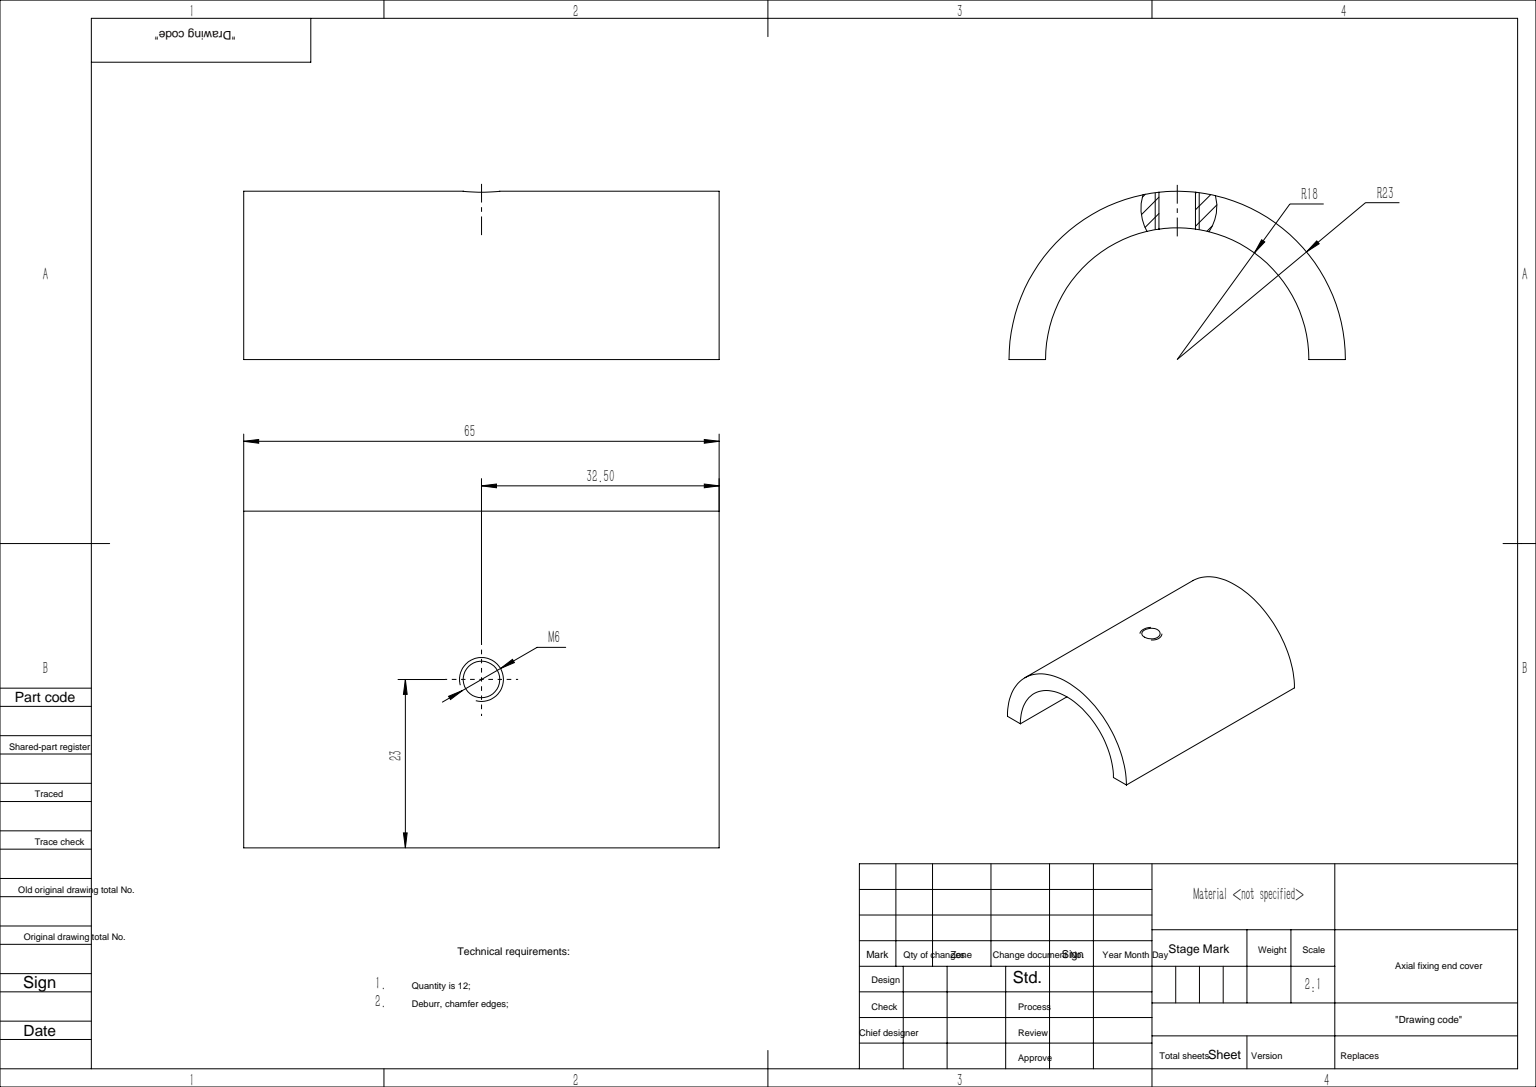
SolidWorks part; units mm, degrees
ref_plane "前视基准面" through (0, 0, 0) normal (0, 0, 1) x (1, 0, 0)
ref_plane "上视基准面" through (0, 0, 0) normal (0, 1, 0) x (1, 0, 0)
ref_plane "右视基准面" through (0, 0, 0) normal (1, 0, 0) x (0, 0, -1)
sketch "草图1" plane through (0, 0, 0) normal (0, 0, 1) x (1, 0, 0)
  line L0 (-23, 0) -> (-18, 0)
  line L1 (18, 0) -> (23, 0)
  arc A0 (18, 0) -> (-18, 0) centre (0, 0) ccw
  arc A1 (23, 0) -> (-23, 0) centre (0, 0) ccw
  circle A2 centre (0, 0) radius 23 construction
  circle A3 centre (0, 0) radius 18 construction
  dimension "D1" = 36
  dimension "D2" = 5
extrude "凸台-拉伸1" add sketch "草图1" against normal blind 65
ref_plane "基准面1" through (23, 0, 0) normal (1, 0, 0) x (0, 0, -1)
hole_wizard "M6 螺纹孔1" positions "3D草图2" profile "草图3" tap size "M6" standard "GB" end condition through all
sketch3d "3D草图2"
  point P0 (0, 23, -32.5)
  dimension "D1" = 32.5
  dimension "D2" = 23
cosmetic thread "孔螺蚊线1"
sketch "草图3" plane through (0, 23, -32.5) normal (1, 0, 0) x (0, 0, 1)
  line L0 (0, 0) -> (0, 23)
  line L1 (0, 23) -> (2.5, 23)
  line L2 (2.5, 23) -> (2.5, 0)
  line L5 (2.5, 0) -> (0, 0)
  line L11 (0, -6.35) -> (0, 107.95) construction
  dimension "通孔螺纹孔钻头直径" = 5
  dimension "通孔螺纹孔钻头深度" = 23
